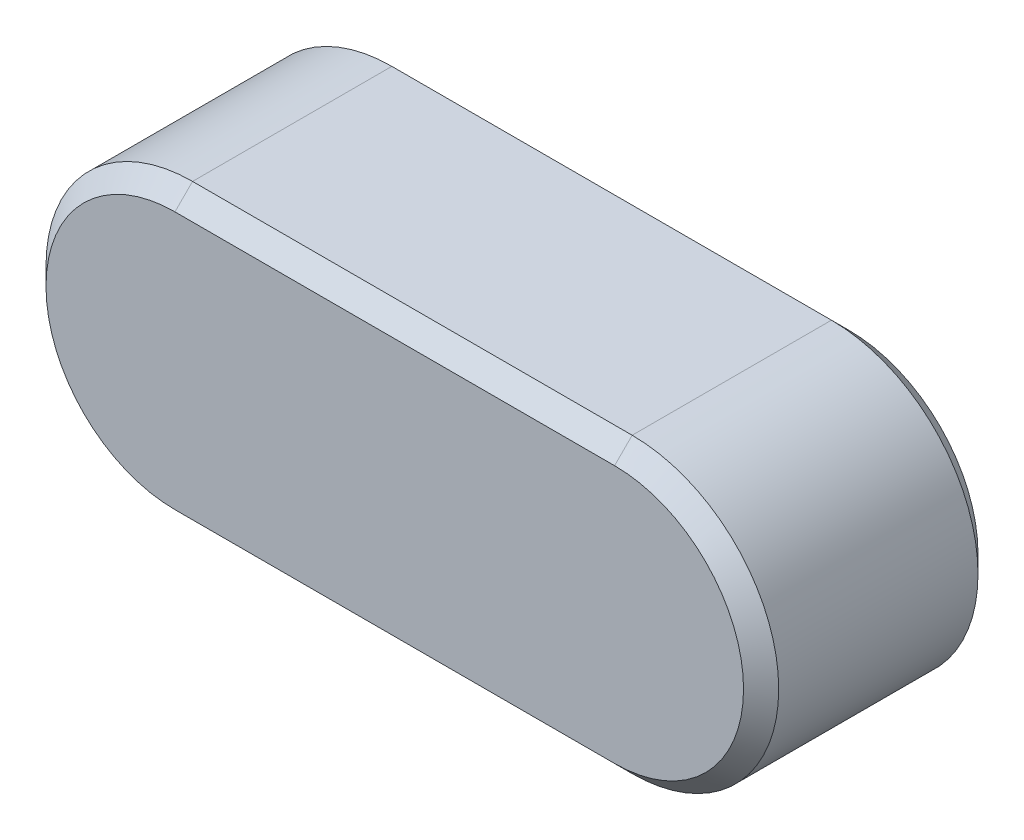
SolidWorks part; units mm, degrees
ref_plane "Front" through (0, 0, 0) normal (0, 0, 1) x (1, 0, 0)
ref_plane "Top" through (0, 0, 0) normal (0, 1, 0) x (1, 0, 0)
ref_plane "Right" through (0, 0, 0) normal (1, 0, 0) x (0, 0, -1)
sketch "Sketch1" plane through (0, 0, 0) normal (0, 0, 1) x (1, 0, 0)
  line L0 (-15, 5) -> (0, 5)
  line L1 (0, -5) -> (-15, -5)
  arc A0 (0, 5) -> (0, -5) centre (0, 0) cw
  arc A1 (-15, -5) -> (-15, 5) centre (-15, 0) cw
  dimension "L" = 25
  dimension "b" = 10
extrude "BaseKey" add sketch "Sketch1" along normal mid plane 8
sketch "Sketch2" plane through (0, 0, 0) normal (0, 0, 1) x (1, 0, 0)
  line L1 (-20, 5) -> (5, 5)
  line L2 (-20, 5) -> (-20, -5)
  line L3 (-20, -5) -> (5, -5)
  line L4 (5, 5) -> (5, -5)
  line L6 (0, -5) -> (-15, -5) construction
  line L7 (-15, 5) -> (0, 5) construction
  arc A2 (0, -5) -> (0, 5) centre (0, 0) ccw construction
  arc A3 (-15, 5) -> (-15, -5) centre (-15, 0) ccw construction
extrude "Extrude1" [suppressed] add sketch "Sketch2" along normal mid plane 8
sketch "Sketch3" plane through (0, 0, 0) normal (0, 0, 1) x (1, 0, 0)
  line L0 (5, 5) -> (-15, 5)
  line L1 (-15, -5) -> (5, -5)
  line L2 (5, -5) -> (5, 5)
  line L5 (-15, 5) -> (0, 5) construction
  arc A0 (-15, 5) -> (-15, -5) centre (-15, 0) ccw
  arc A1 (0, -5) -> (0, 5) centre (0, 0) ccw construction
  arc A4 (-15, 5) -> (-15, -5) centre (-15, 0) ccw construction
extrude "Extrude2" [suppressed] add sketch "Sketch3" along normal mid plane 8
chamfer "Chamfer1" distance 0.6 angle 45 8 edges at (5, 0, -4) (-7.5, -5, -4) (-20, 0, -4) (-7.5, 5, -4) (-20, 0, 4) (-7.5, -5, 4) (5, 0, 4) (-7.5, 5, 4)
equation "\"D1@Extrude1\"=\"h@BaseKey\""
equation "\"D1@Extrude2\"=\"h@BaseKey\""
